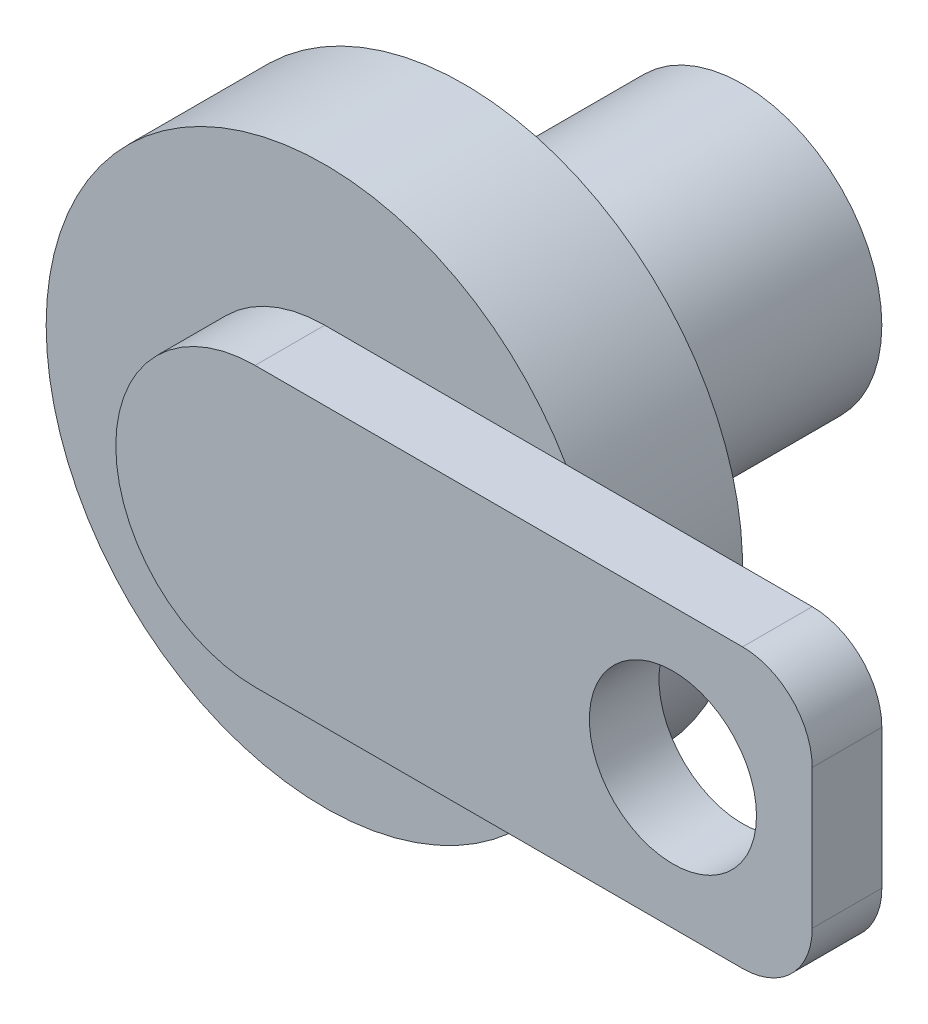
SolidWorks part; units mm, degrees
ref_plane "Front Plane" through (0, 0, 0) normal (0, 0, 1) x (1, 0, 0)
ref_plane "Top Plane" through (0, 0, 0) normal (0, 1, 0) x (1, 0, 0)
ref_plane "Right Plane" through (0, 0, 0) normal (1, 0, 0) x (0, 0, -1)
other "Configuration Table"
sketch "Sketch1" plane through (0, 0, 0) normal (0, 0, 1) x (1, 0, 0)
  line L1 (-50, 20) -> (50, 20)
  line L2 (-50, 20) -> (-50, -20)
  line L3 (-50, -20) -> (50, -20)
  line L4 (50, 20) -> (50, -20)
  line L5 (-50, 20) -> (50, -20) construction
  line L6 (-50, -20) -> (50, 20) construction
  point P0 (0, 0)
  dimension "D1" = 40
  dimension "D2" = 100
extrude "Boss-Extrude1" add sketch "Sketch1" along normal blind 10
sketch "Sketch2" plane through (0, 0, 10) normal (0, 0, 1) x (1, 0, 0)
  line L0 (50, -20) -> (50, 20) construction
  circle A0 centre (30, 0) radius 12
  dimension "D1" = 24
  dimension "D2" = 20
extrude "Cut-Extrude1" cut sketch "Sketch2" against normal blind 10
fillet "Fillet1" radius 10 2 edges at (50, -20, 5) (50, 20, 5)
sketch "Sketch3" plane through (0, 0, 0) normal (0, 0, -1) x (-1, 0, 0)
  line L0 (50, 20) -> (50, -20) construction
  line L1 (30, 20) -> (50, 20)
  line L2 (50, 20) -> (50, 0)
  line L3 (50, 0) -> (50, -20)
  line L4 (50, -20) -> (30, -20)
  arc A0 (30, -20) -> (30, 20) centre (30, 0) ccw
  line M5 (-40, -20) -> (50, -20)
  line M6 (50, -20) -> (50, 20)
  line M7 (50, 20) -> (-40, 20)
extrude "Cut-Extrude2" cut sketch "Sketch3" against normal blind 10 contours A0 M6 M7 | A0 M5 M6
sketch "Sketch4" plane through (0, 0, 0) normal (0, 0, -1) x (-1, 0, 0)
  circle A0 centre (30, 0) radius 20
extrude "Boss-Extrude2" add sketch "Sketch4" along normal blind 60
sketch "Sketch5" plane through (0, 0, 0) normal (0, 0, -1) x (-1, 0, 0)
  circle A0 centre (30, 0) radius 40
  dimension "D1" = 80
extrude "Boss-Extrude3" add sketch "Sketch5" along normal blind 20
